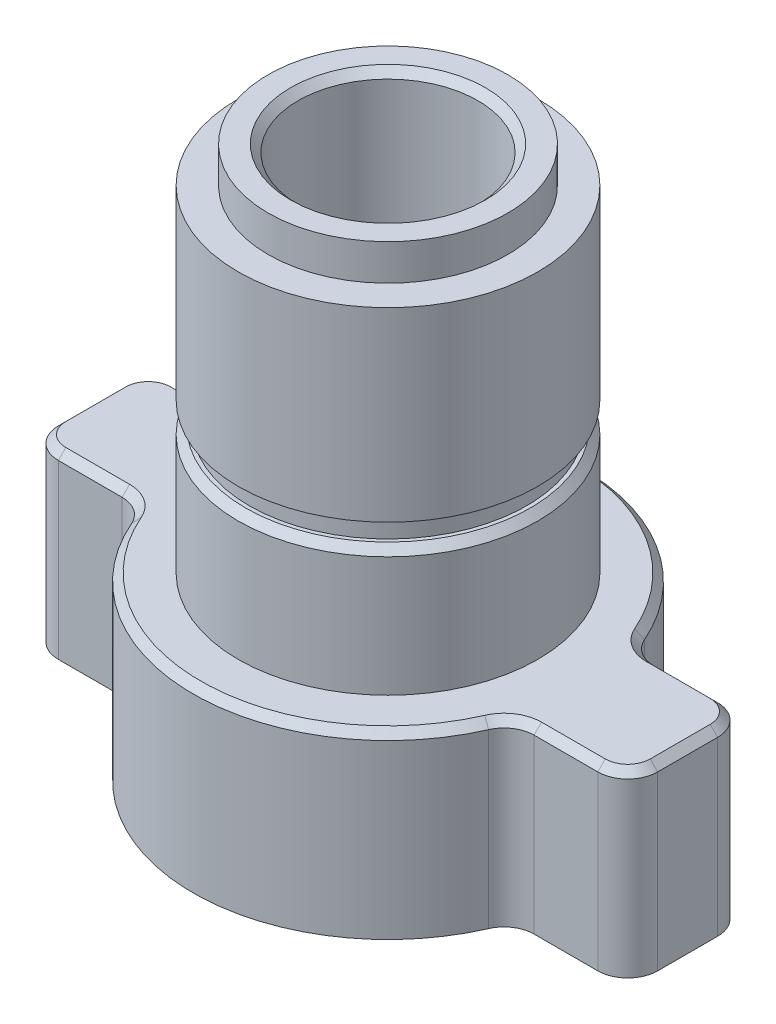
from build123d import *

# Parameters (mm, degrees)
EXTRUDE_1_DEPTH      = 6
SKETCH_2_R           = 5
EXTRUDE_2_DEPTH      = 4.25
SKETCH_3_R           = 4.625
EXTRUDE_3_DEPTH      = 0.75
SKETCH_4_R           = 5
EXTRUDE_M10_1_DEPTH  = 6.2
SKETCH_5_R           = 4
EXTRUDE_5_DEPTH      = 1.2
SKETCH_6_R           = 3
CUT_EXTRUDE_1_DEPTH  = 5
HOLE_WIZARD_M5_1_D   = 4.2
CHAMFER_C0_25_1_SIZE = 0.25


with BuildPart() as part:
    # 草图1 → 凸台-拉伸1 (new body)
    with BuildSketch(Plane(origin=(0, 0, 0), x_dir=(1, 0, 0), z_dir=(0, 1, 0))):
        with BuildLine():
            Line((6.873863542, 2), (9, 2))
            ThreePointArc((9, 2), (9.707106781, 1.707106781), (10, 1))
            Line((10, 1), (10, -1))
            ThreePointArc((10, -1), (9.707106781, -1.707106781), (9, -2))
            Line((9, -2), (6.873863542, -2))
            ThreePointArc((6.873863542, -2), (6.326140985, -2.163339973), (5.957348403, -2.6))
            ThreePointArc((5.957348403, -2.6), (0, -6.5), (-5.957348403, -2.6))
            ThreePointArc((-5.957348403, -2.6), (-6.326140985, -2.163339973), (-6.873863542, -2))
            Line((-6.873863542, -2), (-9, -2))
            ThreePointArc((-9, -2), (-9.707106781, -1.707106781), (-10, -1))
            Line((-10, -1), (-10, 1))
            ThreePointArc((-10, 1), (-9.707106781, 1.707106781), (-9, 2))
            Line((-9, 2), (-6.873863542, 2))
            ThreePointArc((-6.873863542, 2), (-6.326140985, 2.163339973), (-5.957348403, 2.6))
            ThreePointArc((-5.957348403, 2.6), (0, 6.5), (5.957348403, 2.6))
            ThreePointArc((5.957348403, 2.6), (6.326140985, 2.163339973), (6.873863542, 2))
        make_face()
    extrude(amount=EXTRUDE_1_DEPTH)

    # 草图2 → 凸台-拉伸2 (add)
    with BuildSketch(Plane(origin=(0, 6, 0), x_dir=(1, 0, 0), z_dir=(0, 1, 0))):
        with Locations(Location((0, 0, 0), (0, 0, 270))):
            Circle(SKETCH_2_R)
    extrude(amount=EXTRUDE_2_DEPTH)

    # 草图3 → 凸台-拉伸3 (add)
    with BuildSketch(Plane(origin=(0, 10.25, 0), x_dir=(1, 0, 0), z_dir=(0, 1, 0))):
        with Locations(Location((0, 0, 0), (0, 0, 270))):
            Circle(SKETCH_3_R)
    extrude(amount=EXTRUDE_3_DEPTH)

    # 草图4 → M10×1 细牙螺柱 (add)
    with BuildSketch(Plane(origin=(0, 11, 0), x_dir=(1, 0, 0), z_dir=(0, 1, 0))):
        with Locations(Location((0, 0, 0), (0, 0, 270))):
            Circle(SKETCH_4_R)
    extrude(amount=EXTRUDE_M10_1_DEPTH)

    # 草图5 → 凸台-拉伸5 (add)
    with BuildSketch(Plane(origin=(0, 17.2, 0), x_dir=(1, 0, 0), z_dir=(0, 1, 0))):
        with Locations(Location((0, 0, 0), (0, 0, 270))):
            Circle(SKETCH_5_R)
    extrude(amount=EXTRUDE_5_DEPTH)

    # 草图6 → 切除-拉伸1 (cut)
    with BuildSketch(Plane(origin=(0, 18.4, 0), x_dir=(1, 0, 0), z_dir=(0, 1, 0))):
        with Locations(Location((0, 0, 0), (0, 0, 270))):
            Circle(SKETCH_6_R)
    extrude(amount=-CUT_EXTRUDE_1_DEPTH, mode=Mode.SUBTRACT)

    # M5 螺纹孔1 (through all)
    with Locations(Plane(origin=(0, 0, 0), x_dir=(-1, 0, 0), z_dir=(0, -1, 0))):
        with Locations((0, 0)):
            Hole(HOLE_WIZARD_M5_1_D / 2)

    # C0.25 倒角1
    chamfer_c0_25_1_edges = [part.edges().sort_by_distance(p)[0] for p in [
        (-6.326140985, 6, -2.163339973),
        (-7.936931771, 6, -2),
        (-9.707106781, 6, -1.707106781),
        (-10, 6, 0),
        (-9.707106781, 6, 1.707106781),
        (-7.936931771, 6, 2),
        (-6.326140985, 6, 2.163339973),
        (0, 6, 6.5),
        (6.326140985, 6, 2.163339973),
        (0, 10.25, -5),
        (7.936931771, 6, 2),
        (6.326140985, 6, -2.163339973),
        (9.707106781, 6, 1.707106781),
        (10, 6, 0),
        (9.707106781, 6, -1.707106781),
        (7.936931771, 6, -2),
        (0, 18.4, -3),
        (0, 6, -6.5),
    ]]
    chamfer(chamfer_c0_25_1_edges, length=CHAMFER_C0_25_1_SIZE)


solid = part.part
